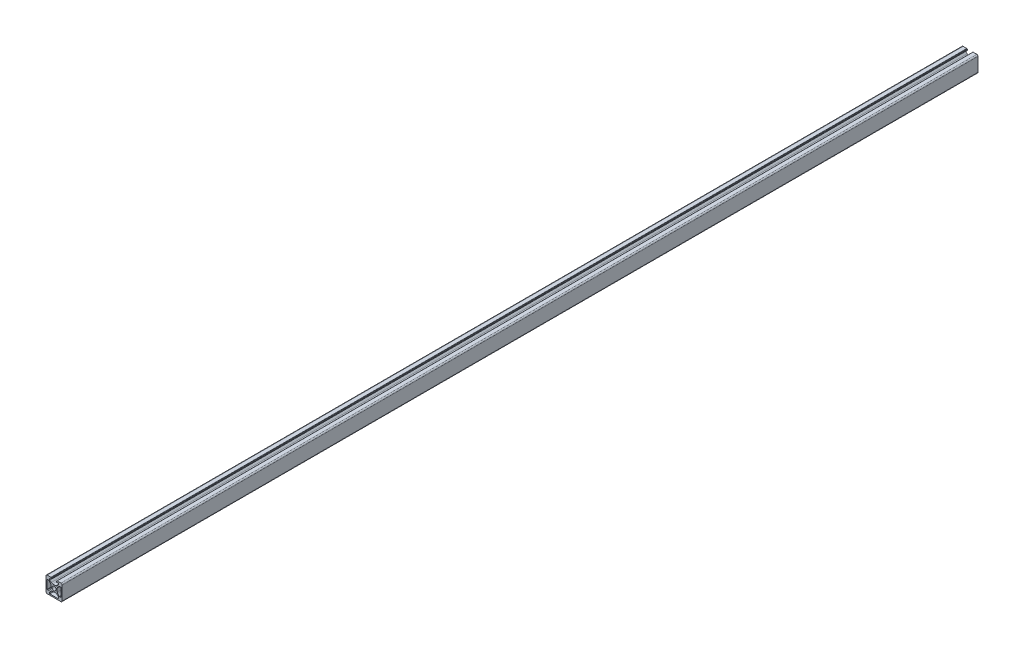
from build123d import *

# Parameters (mm, degrees)
SKETCH_1_R      = 2.5
EXTRUDE_1_DEPTH = 1135


with BuildPart() as part:
    # 草图1 → 凸台-拉伸1 (new body)
    with BuildSketch(Plane.XY):
        with BuildLine():
            Line((-3.425126266, 4.485786438), (-5.412132034, 6.472792206))
            ThreePointArc((-5.412132034, 6.472792206), (-5.47716386, 6.570119211), (-5.5, 6.68492424))
            Line((-5.5, 6.68492424), (-5.5, 7.9))
            ThreePointArc((-5.5, 7.9), (-5.412132034, 8.112132034), (-5.2, 8.2))
            Line((-5.2, 8.2), (-3.4, 8.2))
            ThreePointArc((-3.4, 8.2), (-3.187867966, 8.287867966), (-3.1, 8.5))
            Line((-3.1, 8.5), (-3.1, 9.2))
            ThreePointArc((-3.1, 9.2), (-3.187867966, 9.412132034), (-3.4, 9.5))
            Line((-3.4, 9.5), (-3.6, 9.5))
            Line((-3.6, 9.5), (-3.6, 9.7))
            ThreePointArc((-3.6, 9.7), (-3.687867966, 9.912132034), (-3.9, 10))
            Line((-3.9, 10), (-8.5, 10))
            ThreePointArc((-8.5, 10), (-9.560660172, 9.560660172), (-10, 8.5))
            Line((-10, 8.5), (-10, -8.5))
            ThreePointArc((-10, -8.5), (-9.560660172, -9.560660172), (-8.5, -10))
            Line((-8.5, -10), (8.5, -10))
            ThreePointArc((8.5, -10), (9.560660172, -9.560660172), (10, -8.5))
            Line((10, -8.5), (10, 8.5))
            ThreePointArc((10, 8.5), (9.560660172, 9.560660172), (8.5, 10))
            Line((8.5, 10), (3.9, 10))
            ThreePointArc((3.9, 10), (3.687867966, 9.912132034), (3.6, 9.7))
            Line((3.6, 9.7), (3.6, 9.5))
            Line((3.6, 9.5), (3.4, 9.5))
            ThreePointArc((3.4, 9.5), (3.187867966, 9.412132034), (3.1, 9.2))
            Line((3.1, 9.2), (3.1, 8.5))
            ThreePointArc((3.1, 8.5), (3.187867966, 8.287867966), (3.4, 8.2))
            Line((3.4, 8.2), (5.2, 8.2))
            ThreePointArc((5.2, 8.2), (5.412132034, 8.112132034), (5.5, 7.9))
            Line((5.5, 7.9), (5.5, 6.68492424))
            ThreePointArc((5.5, 6.68492424), (5.47716386, 6.570119211), (5.412132034, 6.472792206))
            Line((5.412132034, 6.472792206), (3.425126266, 4.485786438))
            ThreePointArc((3.425126266, 4.485786438), (2.776279568, 4.052240935), (2.010912703, 3.9))
            Line((2.010912703, 3.9), (-2.010912703, 3.9))
            ThreePointArc((-2.010912703, 3.9), (-2.776279568, 4.052240935), (-3.425126266, 4.485786438))
        make_face()
        Circle(SKETCH_1_R, mode=Mode.SUBTRACT)
        with BuildLine():
            Line((-3.9, 2.010912703), (-3.9, -2.010912703))
            ThreePointArc((-3.9, -2.010912703), (-4.052240935, -2.776279568), (-4.485786438, -3.425126266))
            Line((-4.485786438, -3.425126266), (-6.560660172, -5.5))
            Line((-6.560660172, -5.5), (-8.2, -5.5))
            ThreePointArc((-8.2, -5.5), (-8.412132034, -5.412132034), (-8.5, -5.2))
            Line((-8.5, -5.2), (-8.5, 5.2))
            ThreePointArc((-8.5, 5.2), (-8.412132034, 5.412132034), (-8.2, 5.5))
            Line((-8.2, 5.5), (-6.68492424, 5.5))
            ThreePointArc((-6.68492424, 5.5), (-6.570119211, 5.47716386), (-6.472792206, 5.412132034))
            Line((-6.472792206, 5.412132034), (-4.485786438, 3.425126266))
            ThreePointArc((-4.485786438, 3.425126266), (-4.052240935, 2.776279568), (-3.9, 2.010912703))
        make_face(mode=Mode.SUBTRACT)
        with BuildLine():
            Line((4.485786438, 3.425126266), (6.472792206, 5.412132034))
            ThreePointArc((6.472792206, 5.412132034), (6.570119211, 5.47716386), (6.68492424, 5.5))
            Line((6.68492424, 5.5), (8.2, 5.5))
            ThreePointArc((8.2, 5.5), (8.412132034, 5.412132034), (8.5, 5.2))
            Line((8.5, 5.2), (8.5, -5.2))
            ThreePointArc((8.5, -5.2), (8.412132034, -5.412132034), (8.2, -5.5))
            Line((8.2, -5.5), (6.560660172, -5.5))
            Line((6.560660172, -5.5), (4.485786438, -3.425126266))
            ThreePointArc((4.485786438, -3.425126266), (4.052240935, -2.776279568), (3.9, -2.010912703))
            Line((3.9, -2.010912703), (3.9, 2.010912703))
            ThreePointArc((3.9, 2.010912703), (4.052240935, 2.776279568), (4.485786438, 3.425126266))
        make_face(mode=Mode.SUBTRACT)
        with BuildLine():
            Line((-2.010912703, -3.9), (2.010912703, -3.9))
            ThreePointArc((2.010912703, -3.9), (2.776279568, -4.052240935), (3.425126266, -4.485786438))
            Line((3.425126266, -4.485786438), (5.412132034, -6.472792206))
            ThreePointArc((5.412132034, -6.472792206), (5.47716386, -6.570119211), (5.5, -6.68492424))
            Line((5.5, -6.68492424), (5.5, -8.2))
            ThreePointArc((5.5, -8.2), (5.412132034, -8.412132034), (5.2, -8.5))
            Line((5.2, -8.5), (-5.2, -8.5))
            ThreePointArc((-5.2, -8.5), (-5.412132034, -8.412132034), (-5.5, -8.2))
            Line((-5.5, -8.2), (-5.5, -6.68492424))
            ThreePointArc((-5.5, -6.68492424), (-5.47716386, -6.570119211), (-5.412132034, -6.472792206))
            Line((-5.412132034, -6.472792206), (-3.425126266, -4.485786438))
            ThreePointArc((-3.425126266, -4.485786438), (-2.776279568, -4.052240935), (-2.010912703, -3.9))
        make_face(mode=Mode.SUBTRACT)
    extrude(amount=EXTRUDE_1_DEPTH)


solid = part.part
